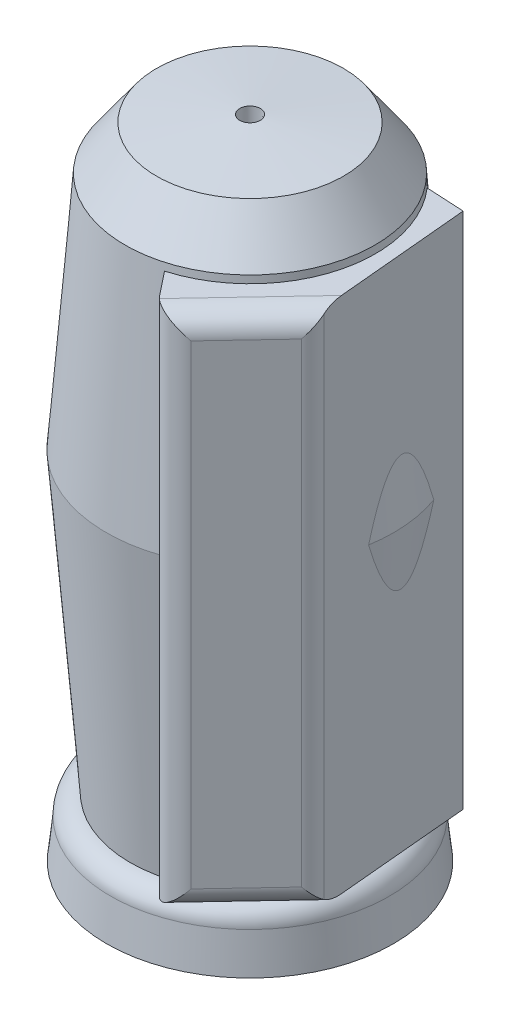
SolidWorks part; units mm, degrees
ref_plane "Front Plane" through (0, 0, 0) normal (0, 0, 1) x (1, 0, 0)
ref_plane "Top Plane" through (0, 0, 0) normal (0, 1, 0) x (1, 0, 0)
ref_plane "Right Plane" through (0, 0, 0) normal (1, 0, 0) x (0, 0, -1)
sketch "Sketch2" plane through (0, 0, 0) normal (0, 0, 1) x (1, 0, 0)
  line L0 (-328.6557, 26.6214) -> (-366.8456, 23.491)
  line L1 (-366.8456, 23.491) -> (-381.2978, 3.3181)
  line L2 (-381.2978, 3.3181) -> (-389.924, -106.756)
  line L3 (-389.924, -106.756) -> (-379.0165, -243.4444)
  line L4 (-379.0165, -243.4444) -> (-328.3181, -239.3988)
  line L5 (-323.9179, -239.0477) -> (-323.9179, 61.0304) construction
  line L6 (-328.6557, 26.6214) -> (-328.6323, 8.1962)
  line L7 (-343.3961, -13.8291) -> (-328.6323, 8.1962)
  line L8 (-328.5619, -47.3068) -> (-328.3181, -239.3988)
  arc A1 (-331.0545, -34.1257) -> (-328.5619, -47.3068) centre (-333.8693, -41.4842) ccw
  ellipse E1 centre (-327.9025, -27.9955) end of major axis (-290.5174, -46.0286) minor radius 6.8909 (-343.3961, -13.8291) -> (-331.0545, -34.1257) ccw
revolve "Revolve1" add sketch "Sketch2" angle 360 about L5
sketch "Sketch3" plane through (0, 0, 0) normal (0, 1, 0) x (1, 0, 0)
  line L0 (-308.6385, 39.5755) -> (-263.1532, 37.1343)
  line L1 (-263.1532, 37.1343) -> (-256.3079, -37.6672)
  line L2 (-256.3079, -37.6672) -> (-291.882, -75.4595)
  line L3 (-291.882, -75.4595) -> (-320.8949, -38.8587)
  line L4 (-308.6385, 39.5755) -> (-273.5947, 2.4979)
  line L5 (-273.5947, 2.4979) -> (-278.656, -19.7342)
  line L6 (-278.656, -19.7342) -> (-298.8487, -43.8673)
  line L7 (-298.8487, -43.8673) -> (-320.8949, -38.8587)
extrude "Boss-Extrude1" add sketch "Sketch3" against normal blind 238
fillet "Fillet1" radius 10 4 edges at (-256.3079, -119, 37.6672) (-274.0949, -238, 56.5634) (-291.882, -119, 75.4595) (-274.0949, 0, 56.5634)
sketch "Sketch5" plane through (0, 0, 0) normal (0, 0, 1) x (1, 0, 0)
  line L0 (-287.9475, -243.4444) -> (-268.8193, -243.4444)
  line L1 (-259.883, -252.3807) -> (-258.0376, -270.3846)
  line L2 (-258.0376, -270.3846) -> (-289.8509, -270.3846)
  line L3 (-289.8509, -270.3846) -> (-287.9475, -243.4444)
  line L4 (-323.9179, 26.6214) -> (-323.9179, 138.1439) construction
  line L5 (-319.1801, 26.6214) -> (-328.6557, 26.6214) construction
  arc A0 (-268.8193, -243.4444) -> (-259.883, -252.3807) centre (-268.8193, -252.3807) cw
revolve "Revolve2" add sketch "Sketch5" angle 360 about L4
